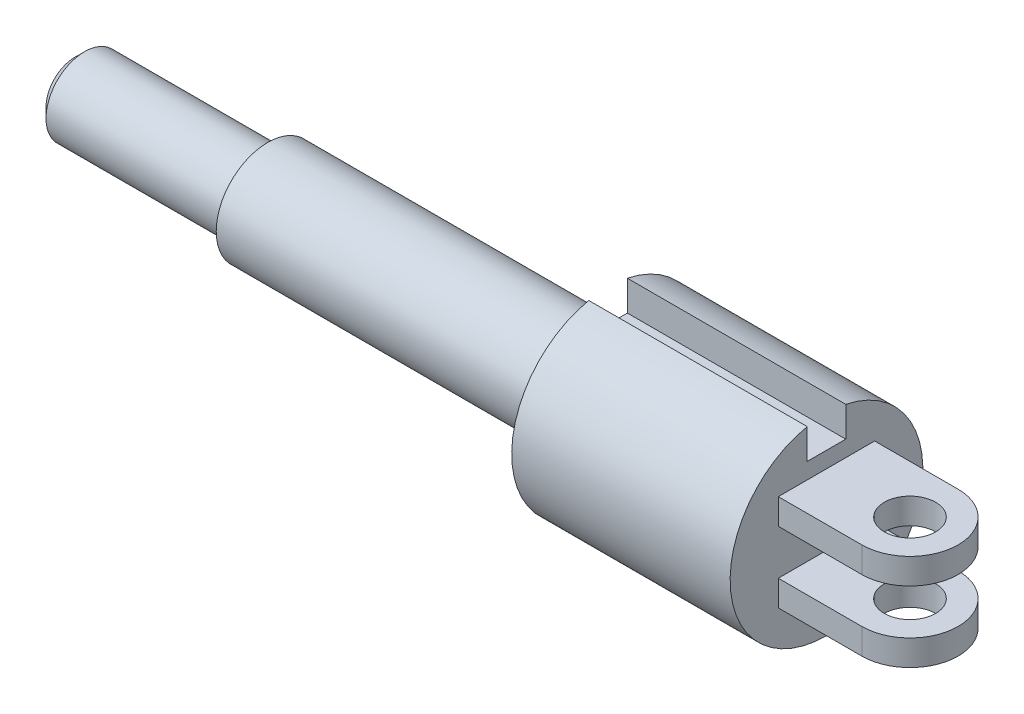
from build123d import *

# Parameters (mm, degrees)
SKETCH_1_W          = 34
SKETCH_1_H          = 30
EXTRUDE_1_DEPTH     = 15
SKETCH_6_R          = 25
SKETCH_6_R_2        = 15
CUT_EXTRUDE_2_DEPTH = 34
CUT_EXTRUDE_START   = 10
SKETCH_2_W          = 34
SKETCH_2_H          = 6
CUT_EXTRUDE_1_DEPTH = 18.184554438
SKETCH_3_R          = 8
EXTRUDE_2_DEPTH     = 53
SKETCH_4_R          = 6
EXTRUDE_3_DEPTH     = 30
CHAMFER_1_SIZE      = 1.5
EXTRUDE_START       = 3.5
SKETCH_5_R          = 4
EXTRUDE_4_DEPTH     = 4


with BuildPart() as part:
    # 草图1 → 凸台-拉伸1 (new, symmetric)
    with BuildSketch(Plane.XY):
        Rectangle(SKETCH_1_W, SKETCH_1_H)
    extrude(amount=EXTRUDE_1_DEPTH, both=True)

    # 草图6 → 切除-拉伸2 (cut)
    with BuildSketch(Plane(origin=(17, 0, 0), x_dir=(0, 0, -1), z_dir=(1, 0, 0))):
        Circle(SKETCH_6_R)
        Circle(SKETCH_6_R_2, mode=Mode.SUBTRACT)
    extrude(amount=-CUT_EXTRUDE_2_DEPTH, mode=Mode.SUBTRACT)

    # 草图2 → 切除-拉伸1 (cut, through all)
    with BuildSketch(Plane(origin=(0, 0, 0), x_dir=(1, 0, 0), z_dir=(0, 1, 0)).offset(CUT_EXTRUDE_START)):
        Rectangle(SKETCH_2_W, SKETCH_2_H)
    extrude(amount=CUT_EXTRUDE_1_DEPTH, mode=Mode.SUBTRACT)

    # 草图3 → 凸台-拉伸2 (add)
    with BuildSketch(Plane.ZY.offset(17)):
        with Locations(Location((0, 0, 0), (0, 0, 180))):
            Circle(SKETCH_3_R)
    extrude(amount=EXTRUDE_2_DEPTH)

    # 草图4 → 凸台-拉伸3 (add)
    with BuildSketch(Plane.ZY.offset(70)):
        Circle(SKETCH_4_R)
    extrude(amount=EXTRUDE_3_DEPTH)

    # 倒角1
    chamfer_1_edges = [part.edges().sort_by_distance(p)[0] for p in [
        (-100, 0, -6),
    ]]
    chamfer(chamfer_1_edges, length=CHAMFER_1_SIZE)

    # 草图5 → 凸台-拉伸4 (add)
    with BuildSketch(Plane(origin=(0, 0, 0), x_dir=(1, 0, 0), z_dir=(0, 1, 0)).offset(EXTRUDE_START)):
        with BuildLine():
            Line((30, -7.5), (17, -7.5))
            Line((17, -7.5), (17, 7.5))
            Line((17, 7.5), (30, 7.5))
            ThreePointArc((30, 7.5), (37.5, 0), (30, -7.5))
        make_face()
        with Locations(Location((30, 0, 0), (0, 0, 270))):
            Circle(SKETCH_5_R, mode=Mode.SUBTRACT)
    extrude_4 = extrude(amount=EXTRUDE_4_DEPTH)

    # 镜向1: 凸台-拉伸4 across plane
    add(extrude_4.mirror(Plane.ZX))


solid = part.part
